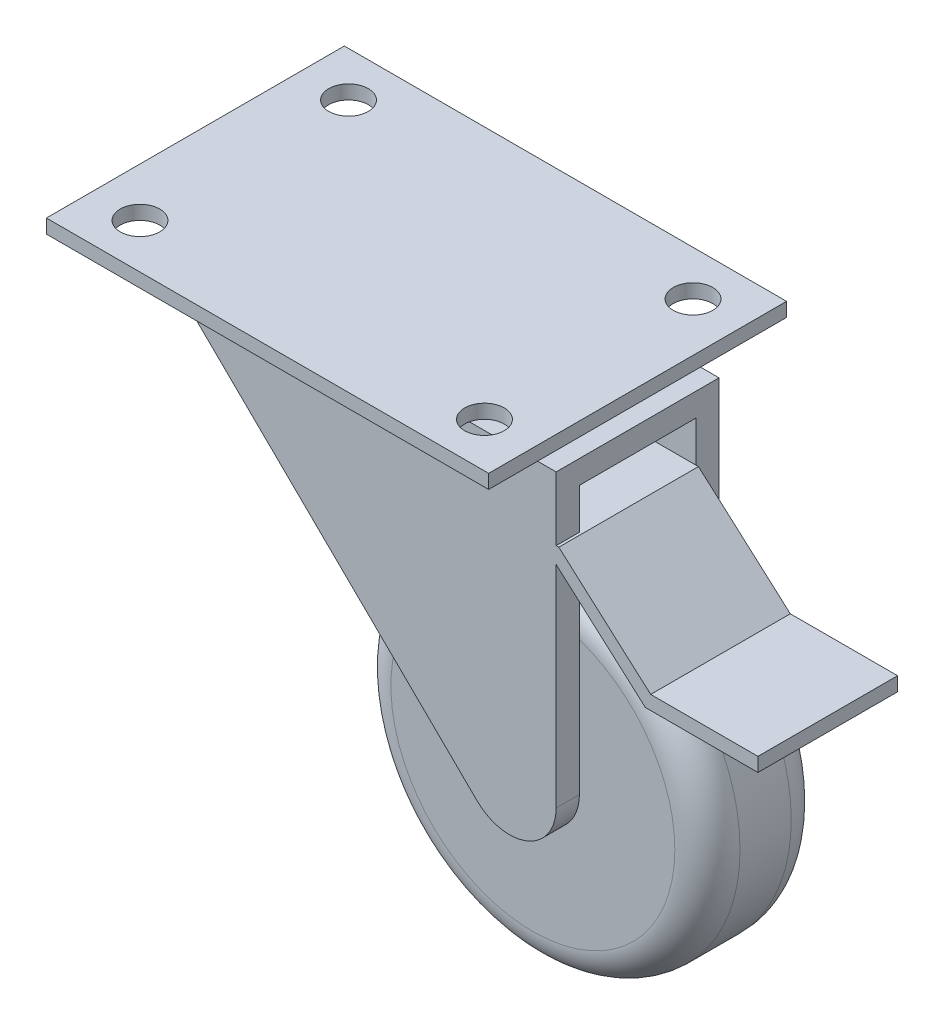
from build123d import *

# Parameters (mm, degrees)
SKETCH_1_R          = 37.5
EXTRUDE_1_DEPTH     = 12.5
FILLET_1_R          = 7
SKETCH_2_R          = 5.411787985
EXTRUDE_2_DEPTH     = 15
EXTRUDE_3_DEPTH     = 5
SKETCH_4_W          = 95
SKETCH_4_H          = 64
EXTRUDE_4_DEPTH     = 3
SKETCH_6_R          = 4.25
CUT_EXTRUDE_1_DEPTH = 141.349563667
SKETCH_9_W          = 92.539395388
SKETCH_9_H          = 8.982437317
CUT_EXTRUDE_2_DEPTH = 121.43878113
SKETCH_10_W         = 82.805159643
SKETCH_10_H         = 35
EXTRUDE_5_DEPTH     = 5
SKETCH_11_R         = 17.5
EXTRUDE_6_DEPTH     = 3.982437317
EXTRUDE_1_2_DEPTH   = 30


with BuildPart() as part:
    # 草图1 → Extrude 1 (new, symmetric)
    with BuildSketch(Plane.XY):
        Circle(SKETCH_1_R)
    extrude(amount=EXTRUDE_1_DEPTH, both=True)

    # 圆角1
    fillet_1_edges = [part.edges().sort_by_distance(p)[0] for p in [
        (-37.5, 0, -12.5),
        (-37.5, 0, 12.5),
    ]]
    fillet(fillet_1_edges, radius=FILLET_1_R)

    # 草图2 → 凸台-拉伸2 (add, symmetric)
    with BuildSketch(Plane.XY):
        Circle(SKETCH_2_R)
    extrude(amount=EXTRUDE_2_DEPTH, both=True)

    # 草图3 → 凸台-拉伸3 (add)
    with BuildSketch(Plane.XY.offset(12.5)):
        with BuildLine():
            Line((-7.008676366, -7.132913542), (-85, 69.5))
            Line((-85, 69.5), (10, 69.5))
            Line((10, 69.5), (10, 0))
            ThreePointArc((10, 0), (3.867378721, -9.221896867), (-7.008676366, -7.132913542))
        make_face()
    extrude_3 = extrude(amount=EXTRUDE_3_DEPTH)

    # 镜向1: 凸台-拉伸3 across plane
    add(extrude_3.mirror(Plane.XY))

    # 草图4 → 凸台-拉伸4 (add)
    with BuildSketch(Plane(origin=(0, 69.5, 0), x_dir=(1, 0, 0), z_dir=(0, 1, 0))):
        with Locations((-37.5, 0)):
            Rectangle(SKETCH_4_W, SKETCH_4_H)
    extrude(amount=-EXTRUDE_4_DEPTH)

    # 草图6 → 切除-拉伸1 (cut, through all)
    with BuildSketch(Plane(origin=(0, 69.5, 0), x_dir=(1, 0, 0), z_dir=(0, 1, 0))):
        with Locations(Location((-0.5, -22.4, 0), (0, 0, 270))):
            Circle(SKETCH_6_R)
        with Locations(Location((-0.5, 22.4, 0), (0, 0, 270))):
            Circle(SKETCH_6_R)
        with Locations(Location((-74.5, 22.4, 0), (0, 0, 270))):
            Circle(SKETCH_6_R)
        with Locations(Location((-74.5, -22.4, 0), (0, 0, 270))):
            Circle(SKETCH_6_R)
    extrude(amount=-CUT_EXTRUDE_1_DEPTH, mode=Mode.SUBTRACT)

    # 草图9 → 切除-拉伸2 (cut, through all)
    with BuildSketch(Plane.XY.offset(17.5)):
        with Locations((-36.269697694, 62.008781341)):
            Rectangle(SKETCH_9_W, SKETCH_9_H)
    extrude(amount=-CUT_EXTRUDE_2_DEPTH, mode=Mode.SUBTRACT)


with BuildPart() as cut_extrude_2_piece_1:
    # of the separate pieces the step leaves, piece 1, a body of its own (cut_extrude_2_pieces)
    add(part.part.solids().sort_by_distance((37.5, 0, -5.5))[0])

    # 草图10 → 凸台-拉伸5 (add)
    with BuildSketch(Plane(origin=(0, 57.517562683, 0), x_dir=(1, 0, 0), z_dir=(0, 1, 0))):
        with Locations((-31.402579822, 0)):
            Rectangle(SKETCH_10_W, SKETCH_10_H)
    extrude(amount=EXTRUDE_5_DEPTH)



with BuildPart() as cut_extrude_2_piece_2:
    # of the separate pieces the step leaves, piece 2, a body of its own (cut_extrude_2_pieces)
    add(part.part.solids().sort_by_distance((10, 66.5, 32))[0])


with BuildPart() as cut_extrude_2_piece_1_1:
    add(cut_extrude_2_piece_1.part)

    add(cut_extrude_2_piece_2.part)  # 凸台-拉伸6 merges 切除-拉伸2 piece 2
    # 草图11 → 凸台-拉伸6 (add)
    with BuildSketch(Plane(origin=(0, 62.517562683, 0), x_dir=(1, 0, 0), z_dir=(0, 1, 0))):
        with Locations(Location((-31.402579821, 0, 0), (0, 0, 270))):
            Circle(SKETCH_11_R)
    extrude(amount=EXTRUDE_6_DEPTH)

    # 草图8 → Extrude 1 2 (add)
    with BuildSketch(Plane.XY.offset(17.5)):
        Polygon((-19.25, 45.79201997), (9.430275915, 45.79201997), (29.164495175, 28.274139716), (53.347206554, 28.274139716), (53.347206554, 31.274139716), (30.303943346, 31.274139716), (10.569724085, 48.79201997), (-19.25, 48.79201997), align=None)
    extrude(amount=-EXTRUDE_1_2_DEPTH)


solid = cut_extrude_2_piece_1_1.part
